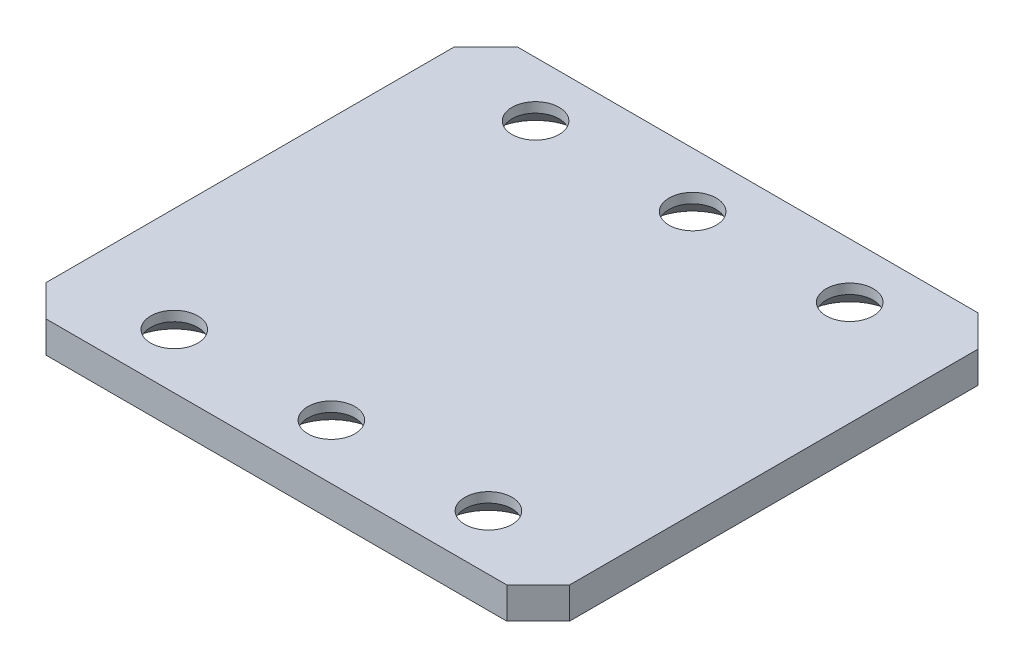
SolidWorks part; units mm, degrees
material "S45C"
ref_plane "前视基准面" through (0, 0, 0) normal (0, 0, 1) x (1, 0, 0)
ref_plane "上视基准面" through (0, 0, 0) normal (0, 1, 0) x (1, 0, 0)
ref_plane "右视基准面" through (0, 0, 0) normal (1, 0, 0) x (0, 0, -1)
sketch "草图1" plane through (0, 0, 0) normal (0, 1, 0) x (1, 0, 0)
  line L5 (-25, 22.5) -> (25, 22.5)
  line L6 (-25, 22.5) -> (-25, -22.5)
  line L7 (-25, -22.5) -> (25, -22.5)
  line L8 (25, 22.5) -> (25, -22.5)
  line L9 (-25, 22.5) -> (25, -22.5) construction
  line L10 (-25, -22.5) -> (25, 22.5) construction
  point P0 (0, 0)
  dimension "D1" = 50
  dimension "D2" = 45
extrude "凸台-拉伸1" add sketch "草图1" along normal blind 3
hole_wizard "打孔尺寸(%根据)开槽半沉头木螺钉的类型1" positions "草图2" profile "草图3" countersink size "M4" standard "GB"
sketch "草图2" plane through (0, 0, 0) normal (0, -1, 0) x (-1, 0, 0)
  point P0 (15, 17.25)
  point P3 (0, 17.25)
  point P6 (-15, 17.25)
  point P9 (-15, -17.25)
  point P12 (0, -17.25)
  point P15 (15, -17.25)
sketch "草图3" plane through (-15, 0, -17.25) normal (1, 0, 0) x (0, 0, -1)
  line L0 (0, 0) -> (0, 13.7519)
  line L1 (0, 13.7519) -> (2.25, 12.4)
  line L2 (2.25, 12.4) -> (2.25, 2.05)
  line L3 (2.25, 2.05) -> (4.3, 0)
  line L5 (4.3, 0) -> (0, 0)
  line L6 (-2.25, 2.05) -> (-4.3, 0) construction
  line L10 (0, 13.7519) -> (-2.25, 12.4) construction
  line L11 (0, -6.35) -> (0, 107.95) construction
  dimension "孔直径" = 4.5
  dimension "孔深度" = 12.4
  dimension "近端锥形沉头孔直径" = 8.6
  dimension "近端锥形沉头孔角度" = 90
  dimension "导头角度" = 118
chamfer "倒角1" distance 3 angle 45 4 edges at (-25, 1.5, -22.5) (25, 1.5, -22.5) (25, 1.5, 22.5) (-25, 1.5, 22.5)
